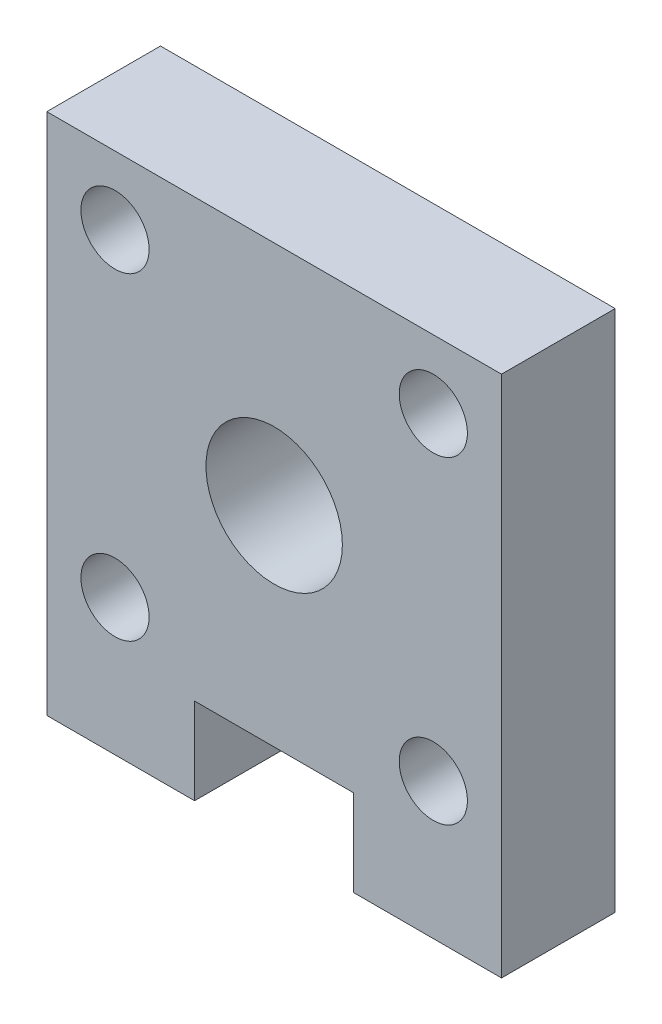
from build123d import *

# Parameters (mm, degrees)
SKETCH1_R           = 3
SKETCH1_R_2         = 1.5
BOSS_EXTRUDE1_DEPTH = 5


with BuildPart() as part:
    # Sketch1 → Boss-Extrude1 (new body)
    with BuildSketch(Plane.XY):
        Polygon((-10, -10), (-10, 10), (-5, 10), (5, 10), (10, 10), (10, -10), (10, -13), (3.5, -13), (3.5, -9.2), (-3.5, -9.2), (-3.5, -13), (-10, -13), align=None)
        Circle(SKETCH1_R, mode=Mode.SUBTRACT)
        with Locations((-7, 7)):
            Circle(SKETCH1_R_2, mode=Mode.SUBTRACT)
        with Locations((7, 7)):
            Circle(SKETCH1_R_2, mode=Mode.SUBTRACT)
        with Locations((7, -7)):
            Circle(SKETCH1_R_2, mode=Mode.SUBTRACT)
        with Locations((-7, -7)):
            Circle(SKETCH1_R_2, mode=Mode.SUBTRACT)
    extrude(amount=BOSS_EXTRUDE1_DEPTH)


solid = part.part
